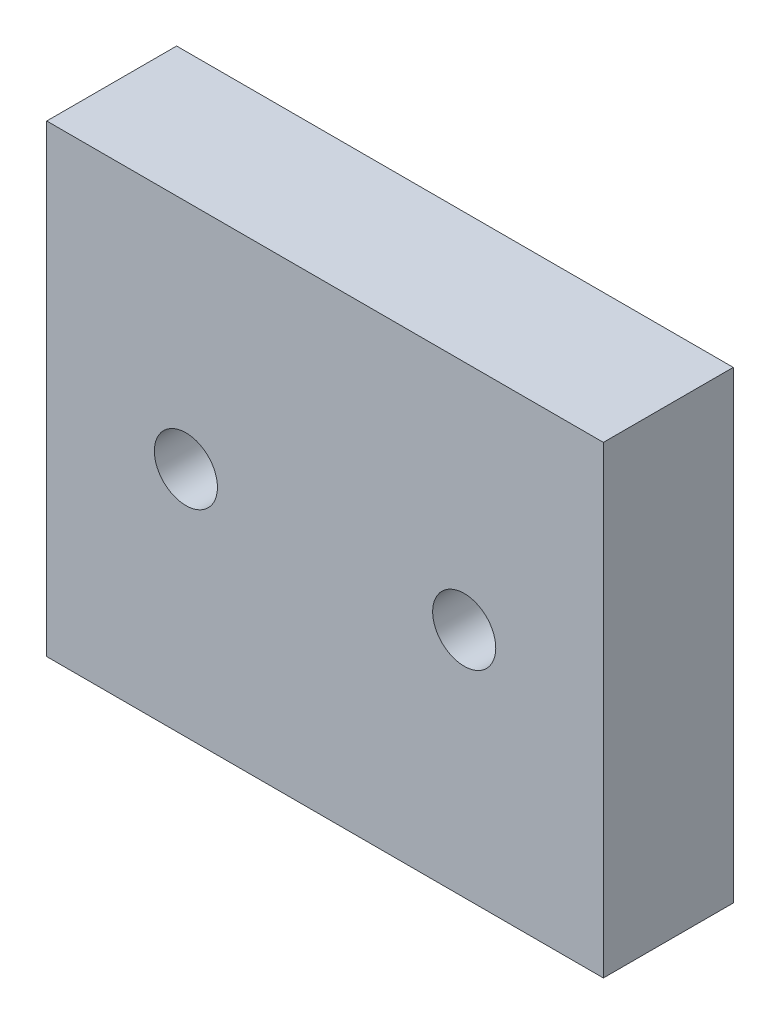
from build123d import *

# Parameters (mm, degrees)
SKETCH1_W             = 60
SKETCH1_H             = 50
BOSS_EXTRUDE1_DEPTH   = 14
M8_TAPPED_HOLE1_D     = 6.8
M8_TAPPED_HOLE1_DEPTH = 19.75
M8_TAPPED_HOLE1_TIP   = 2.042926105


with BuildPart() as part:
    # Sketch1 → Boss-Extrude1 (new body)
    with BuildSketch(Plane.XY):
        Rectangle(SKETCH1_W, SKETCH1_H)
    extrude(amount=BOSS_EXTRUDE1_DEPTH)

    # M8 Tapped Hole1
    with Locations(Plane.XY.offset(14)):
        with Locations((-15, 0), (15, 0)):
            Hole(M8_TAPPED_HOLE1_D / 2, depth=M8_TAPPED_HOLE1_DEPTH)
            with Locations((0, 0, -(M8_TAPPED_HOLE1_DEPTH + M8_TAPPED_HOLE1_TIP / 2))):  # 118° drill point
                Cone(0, M8_TAPPED_HOLE1_D / 2, M8_TAPPED_HOLE1_TIP, mode=Mode.SUBTRACT)


solid = part.part
